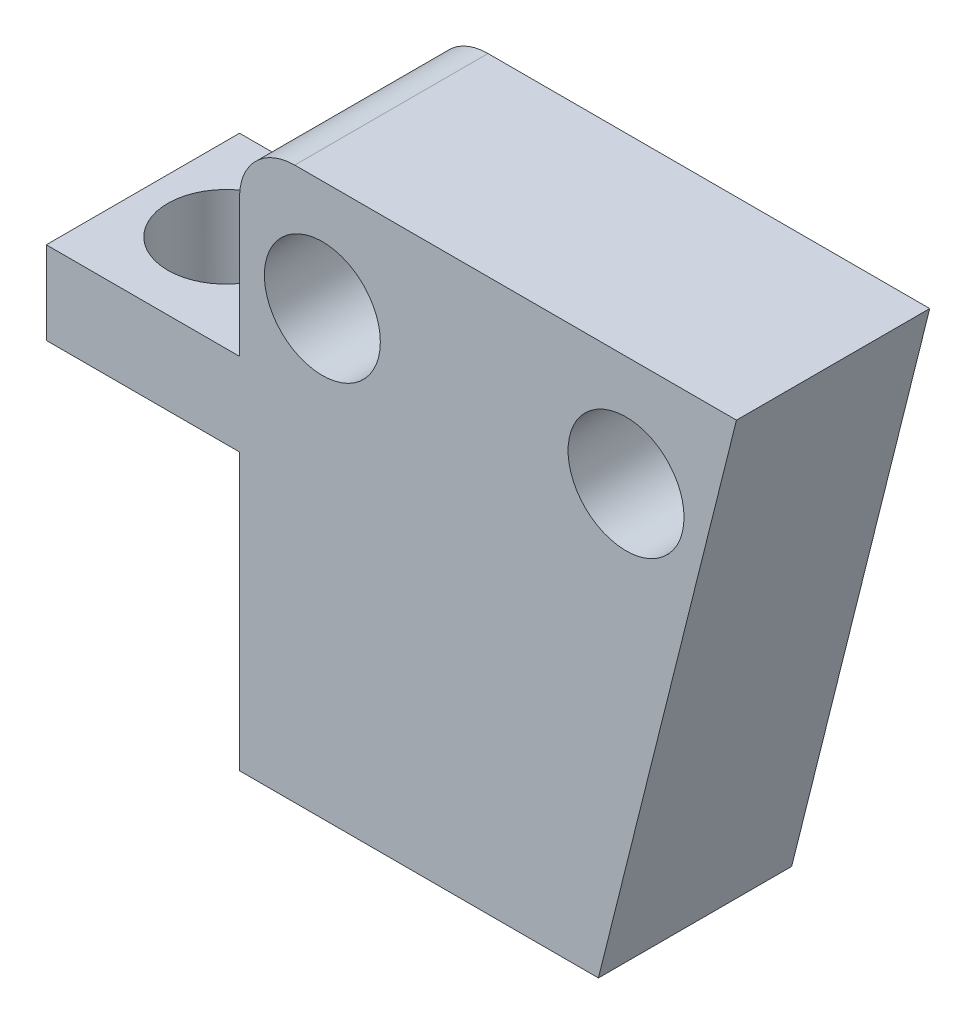
from build123d import *

# Parameters (mm, degrees)
SKETCH2_R           = 2.667
BOSS_EXTRUDE1_DEPTH = 8.89
SKETCH3_R           = 2.667
CUT_EXTRUDE1_DEPTH  = 30.566734686
FILLET1_R           = 2.54
SCALE1_SCALE        = 2


with BuildPart() as part:
    # Sketch2 → Boss-Extrude1 (new body)
    with BuildSketch(Plane.XY):
        Polygon((0, 0), (0, 12.7), (-8.89, 12.7), (-8.89, 16.51), (0, 16.51), (0, 25.4), (22.86, 25.4), (16.51, 0), align=None)
        with Locations((3.81, 20.32)):
            Circle(SKETCH2_R, mode=Mode.SUBTRACT)
        with Locations((17.78, 20.32)):
            Circle(SKETCH2_R, mode=Mode.SUBTRACT)
    extrude(amount=BOSS_EXTRUDE1_DEPTH)

    # Sketch3 → Cut-Extrude1 (cut, through all)
    with BuildSketch(Plane(origin=(0, 16.51, 0), x_dir=(1, 0, 0), z_dir=(0, 1, 0))):
        with Locations(Location((-5.08, -4.445, 0), (0, 0, 270))):
            Circle(SKETCH3_R)
    extrude(amount=-CUT_EXTRUDE1_DEPTH, mode=Mode.SUBTRACT)

    # Fillet1
    fillet1_edges = [part.edges().sort_by_distance(p)[0] for p in [
        (0, 25.4, 4.445),
    ]]
    fillet(fillet1_edges, radius=FILLET1_R)


with BuildPart() as part_1:
    # Scale1: scaled about (0, 0, 0)
    add(part.part.scale(SCALE1_SCALE))


solid = part_1.part
